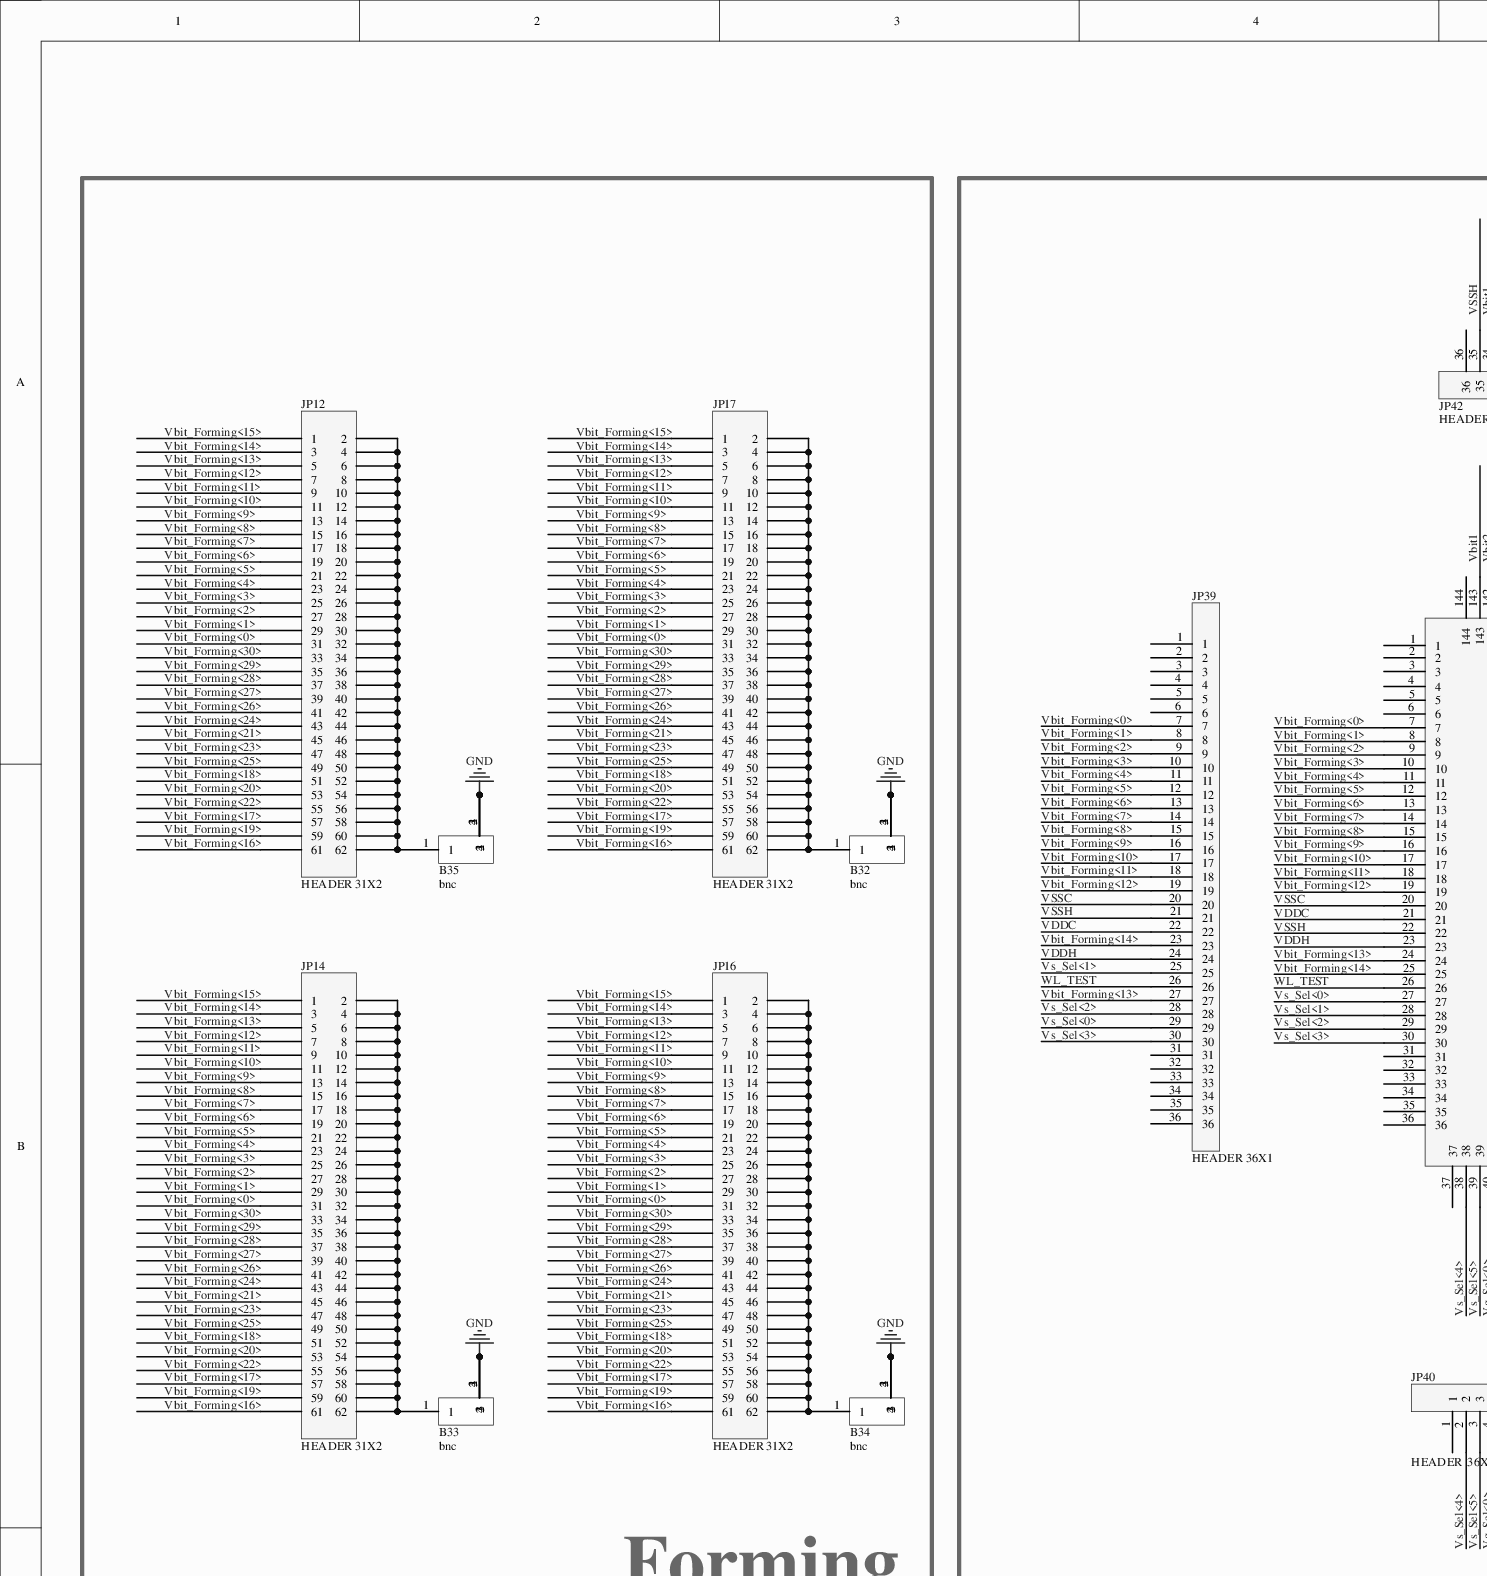
[diagram p0: MISC62794-8.SchDoc, top left]
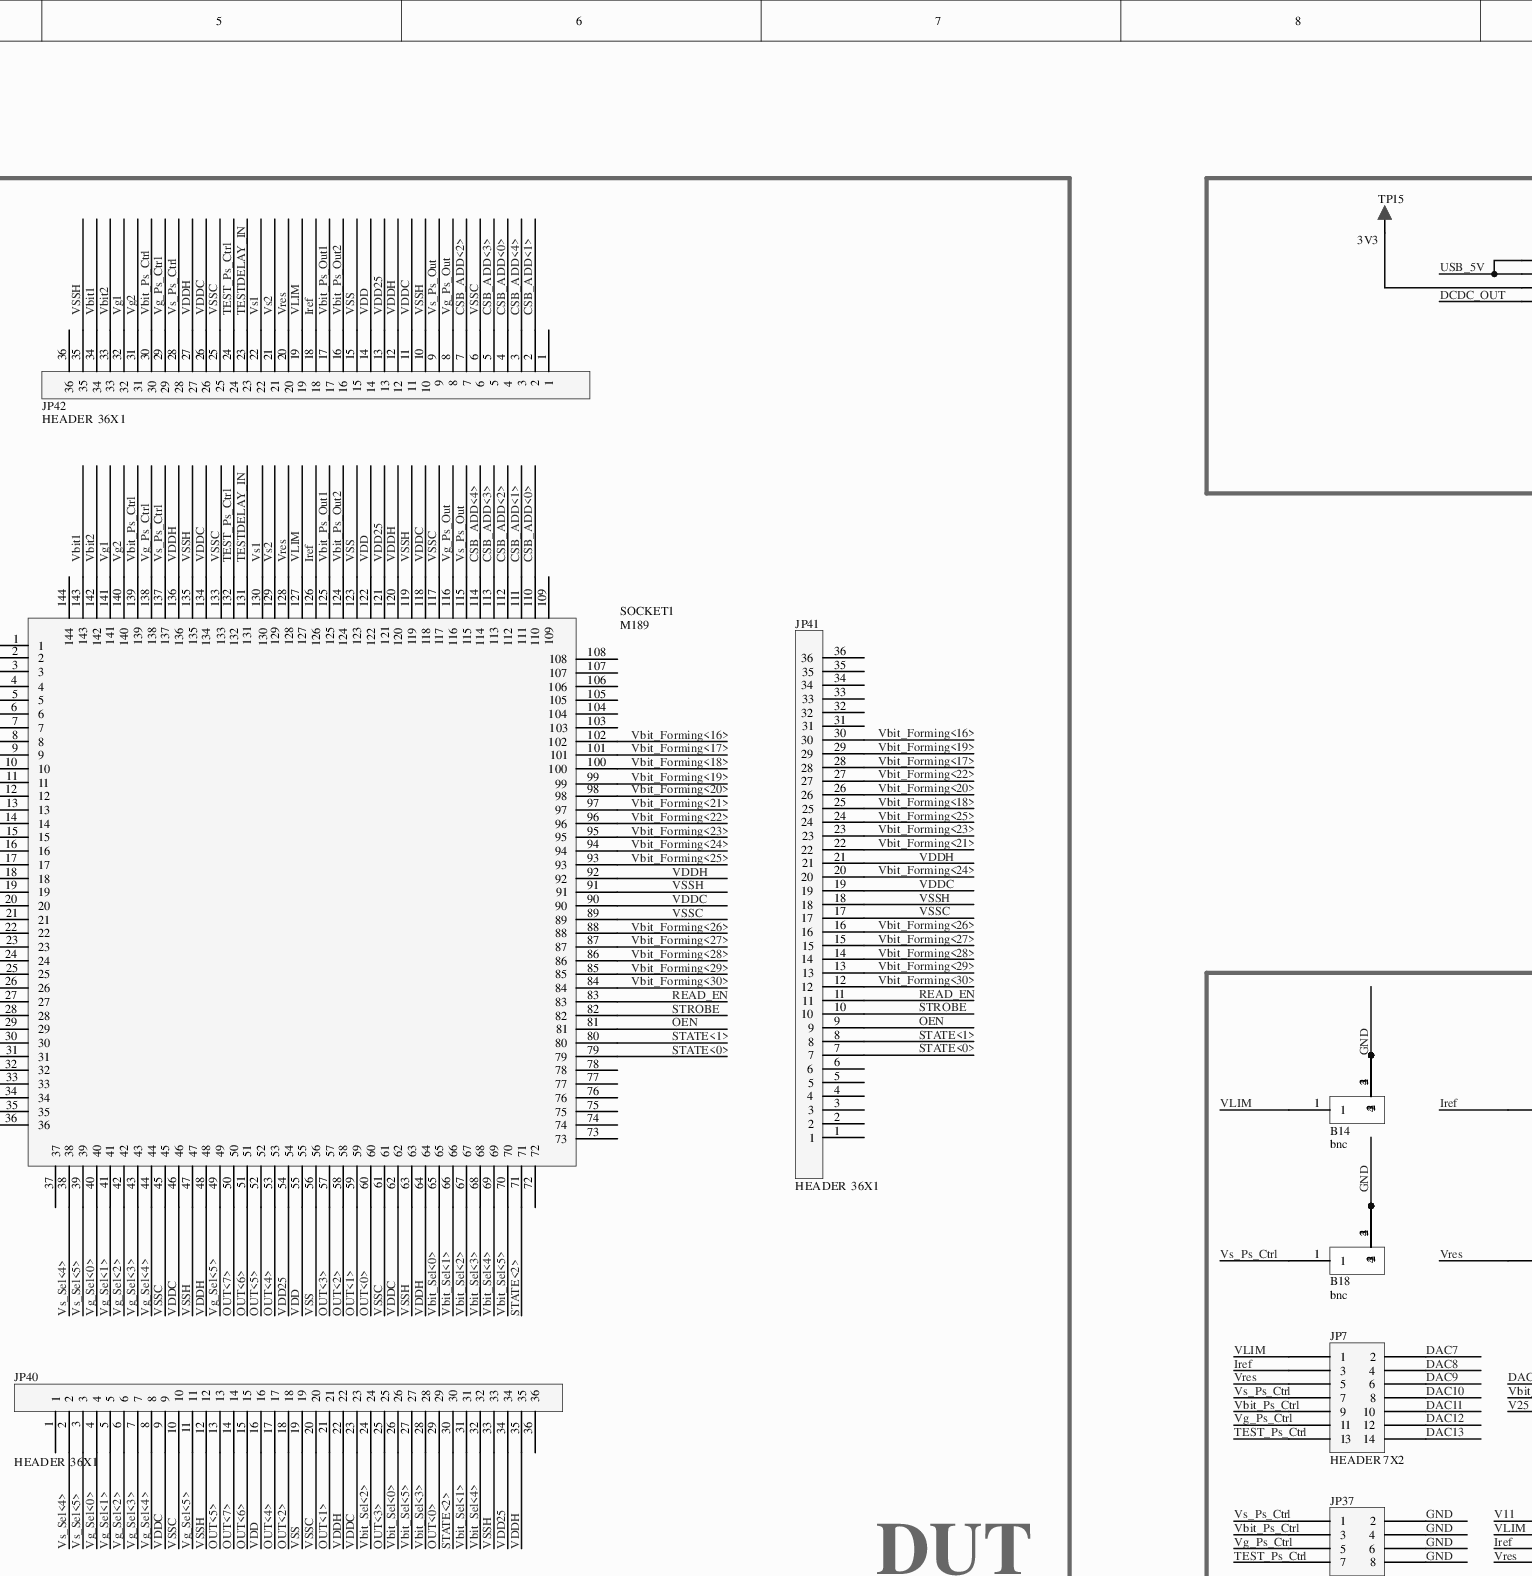
[diagram p1: MISC62794-8.SchDoc, top middle]
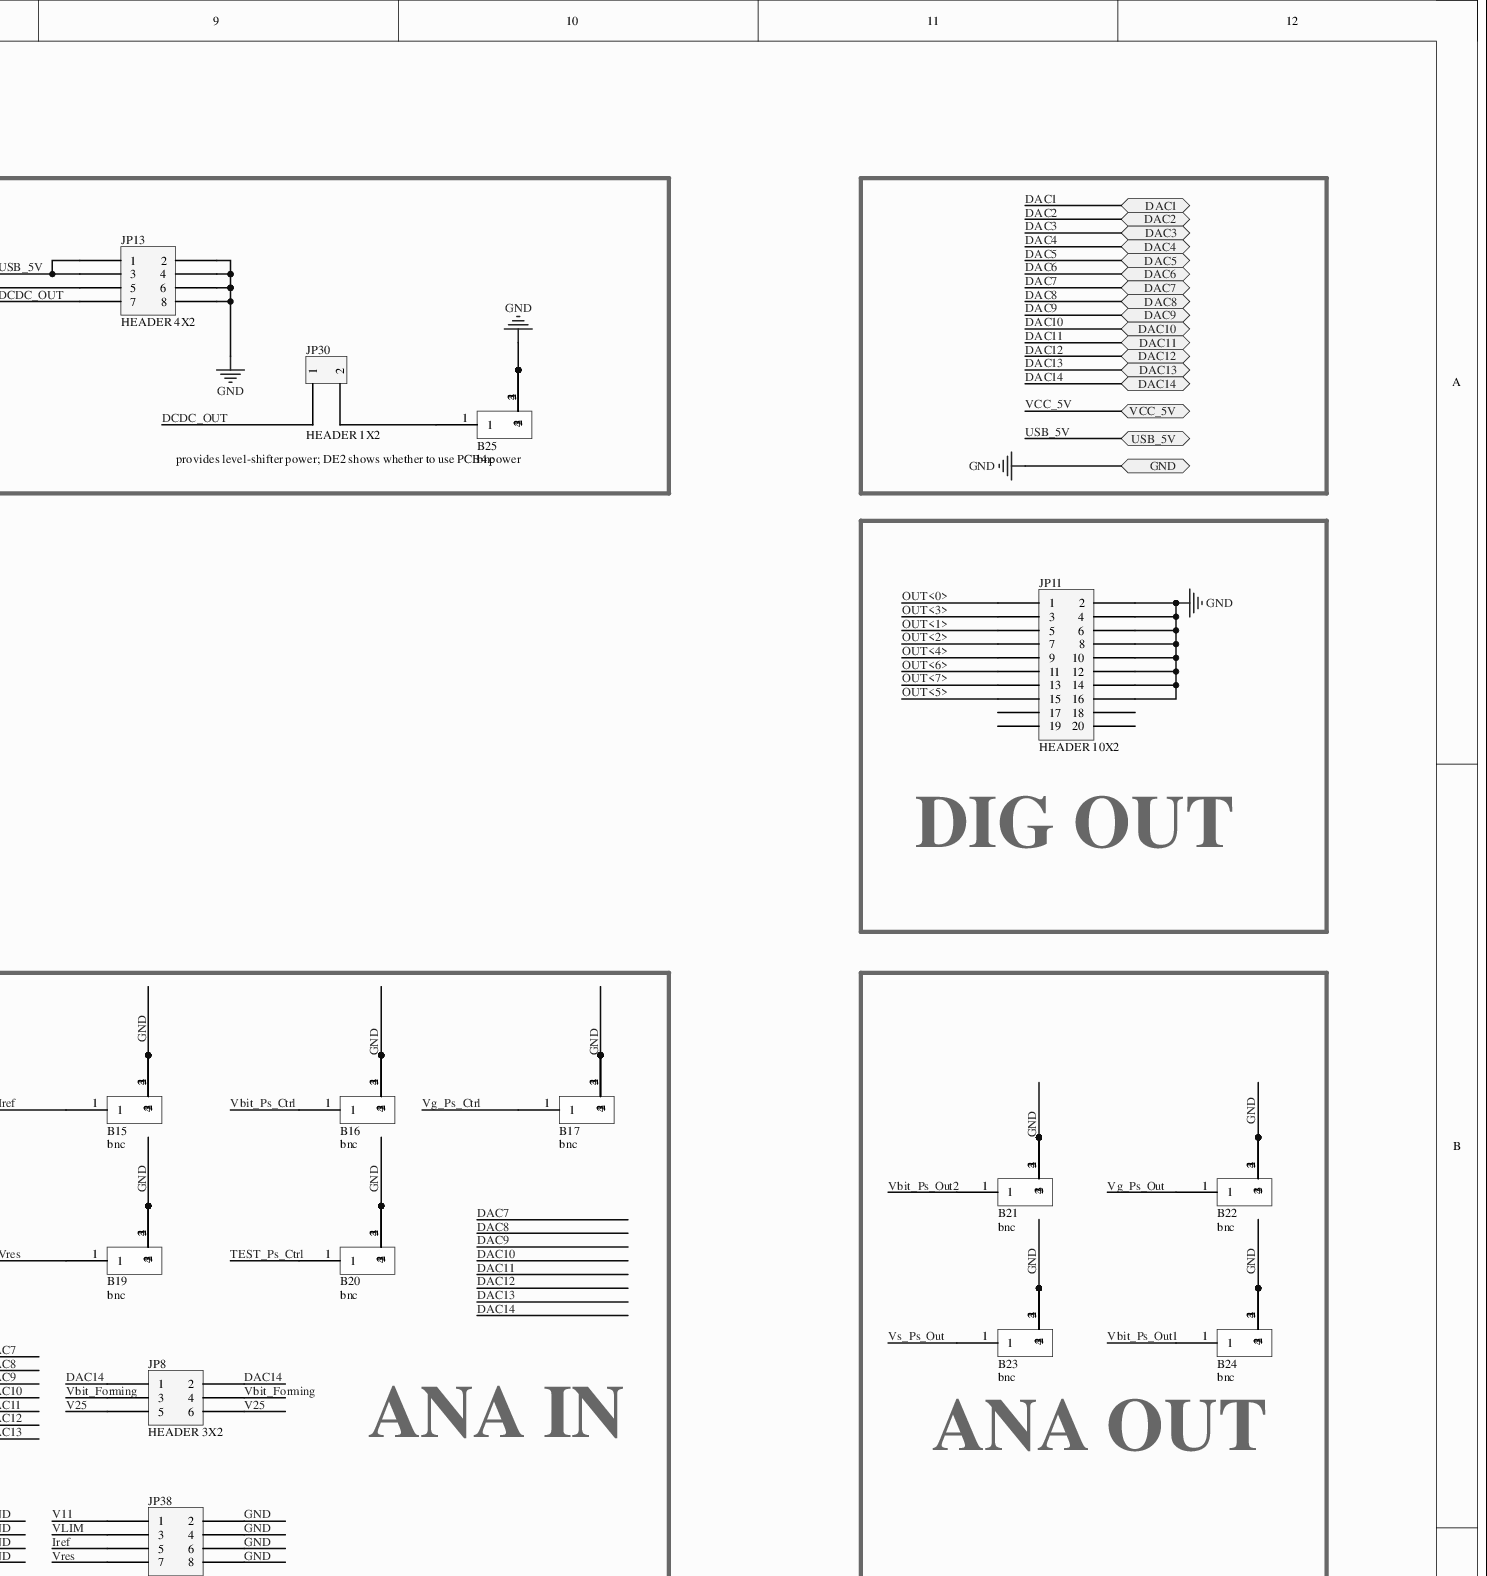
[diagram p2: MISC62794-8.SchDoc, top right]
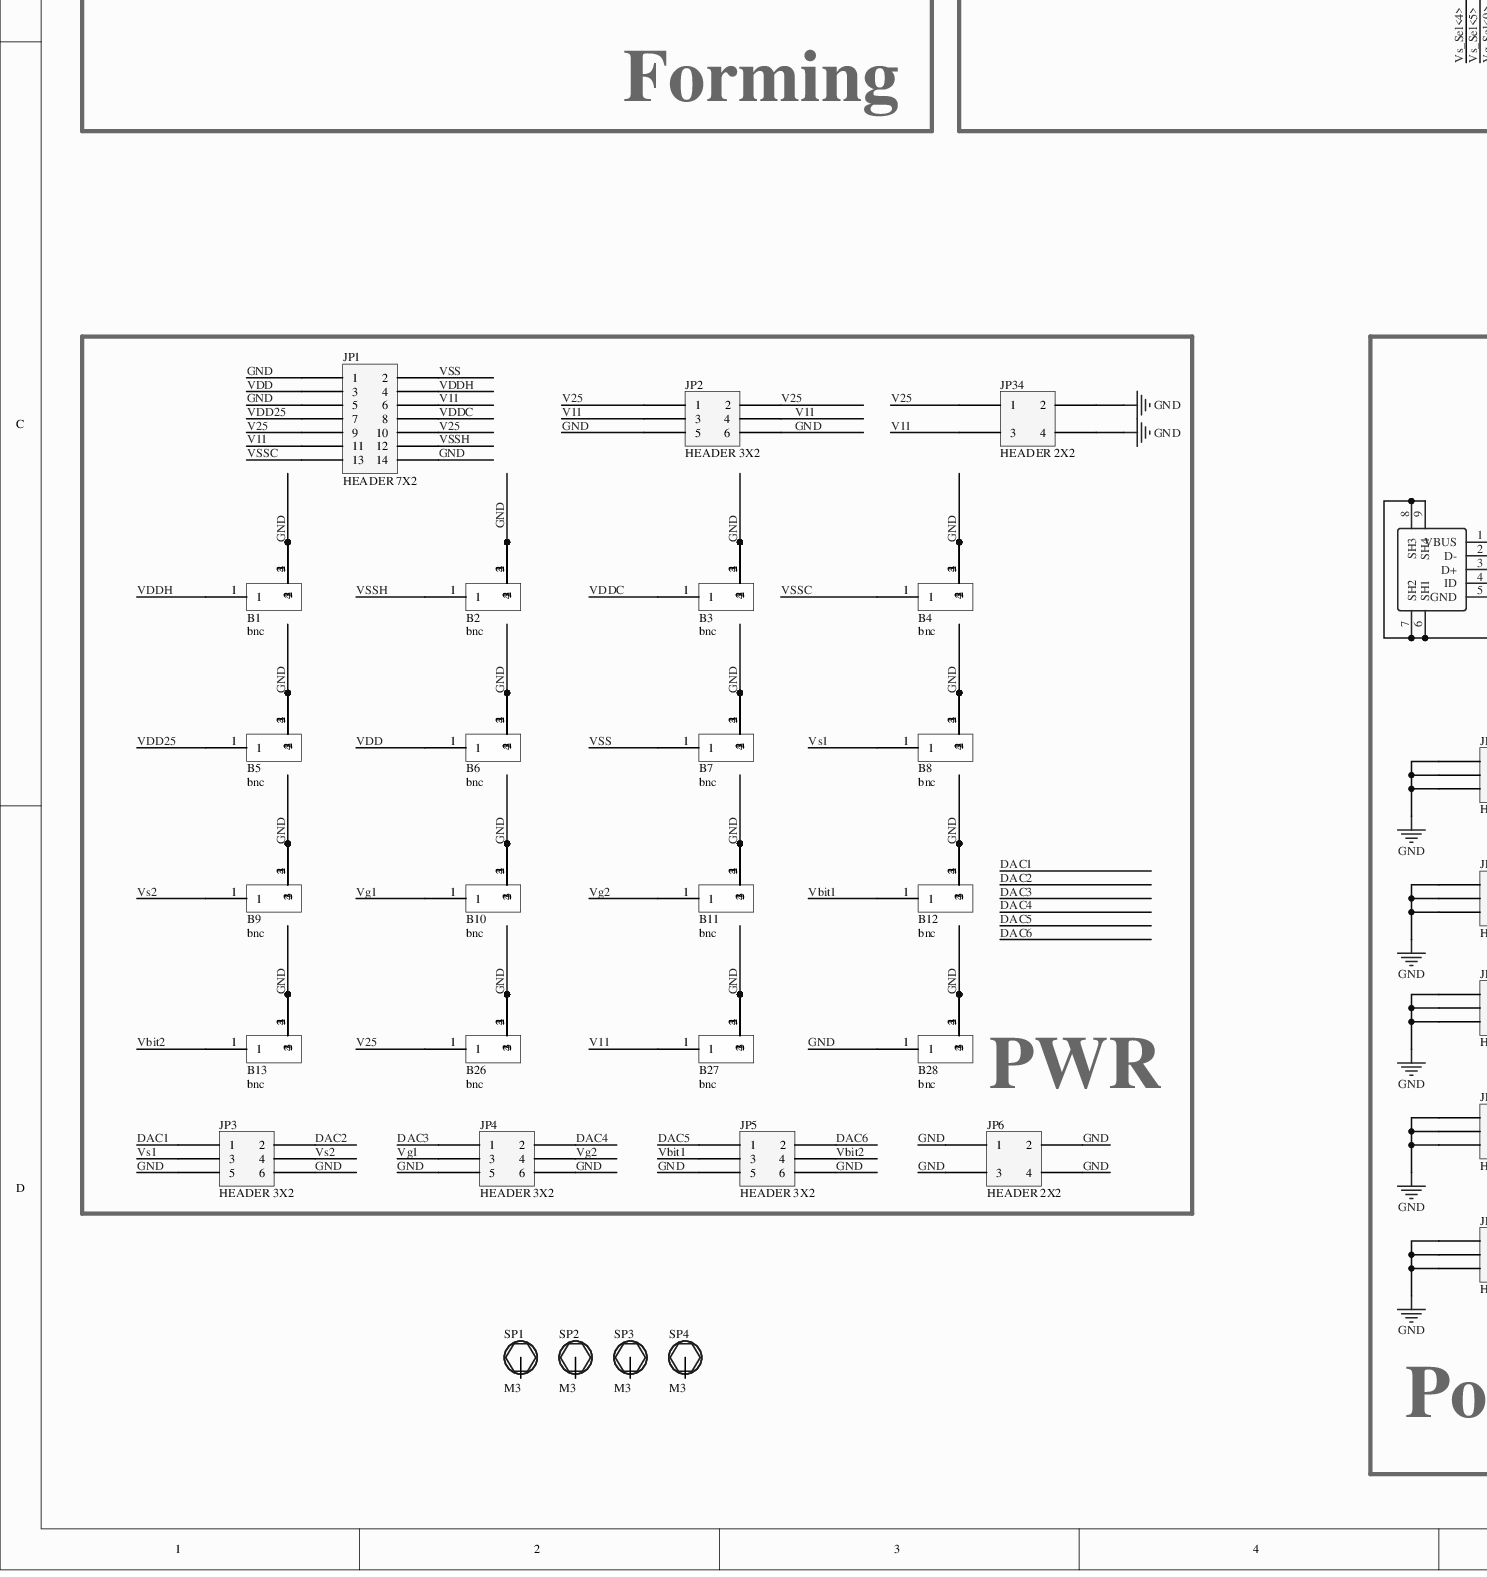
[diagram p3: MISC62794-8.SchDoc, bottom left]
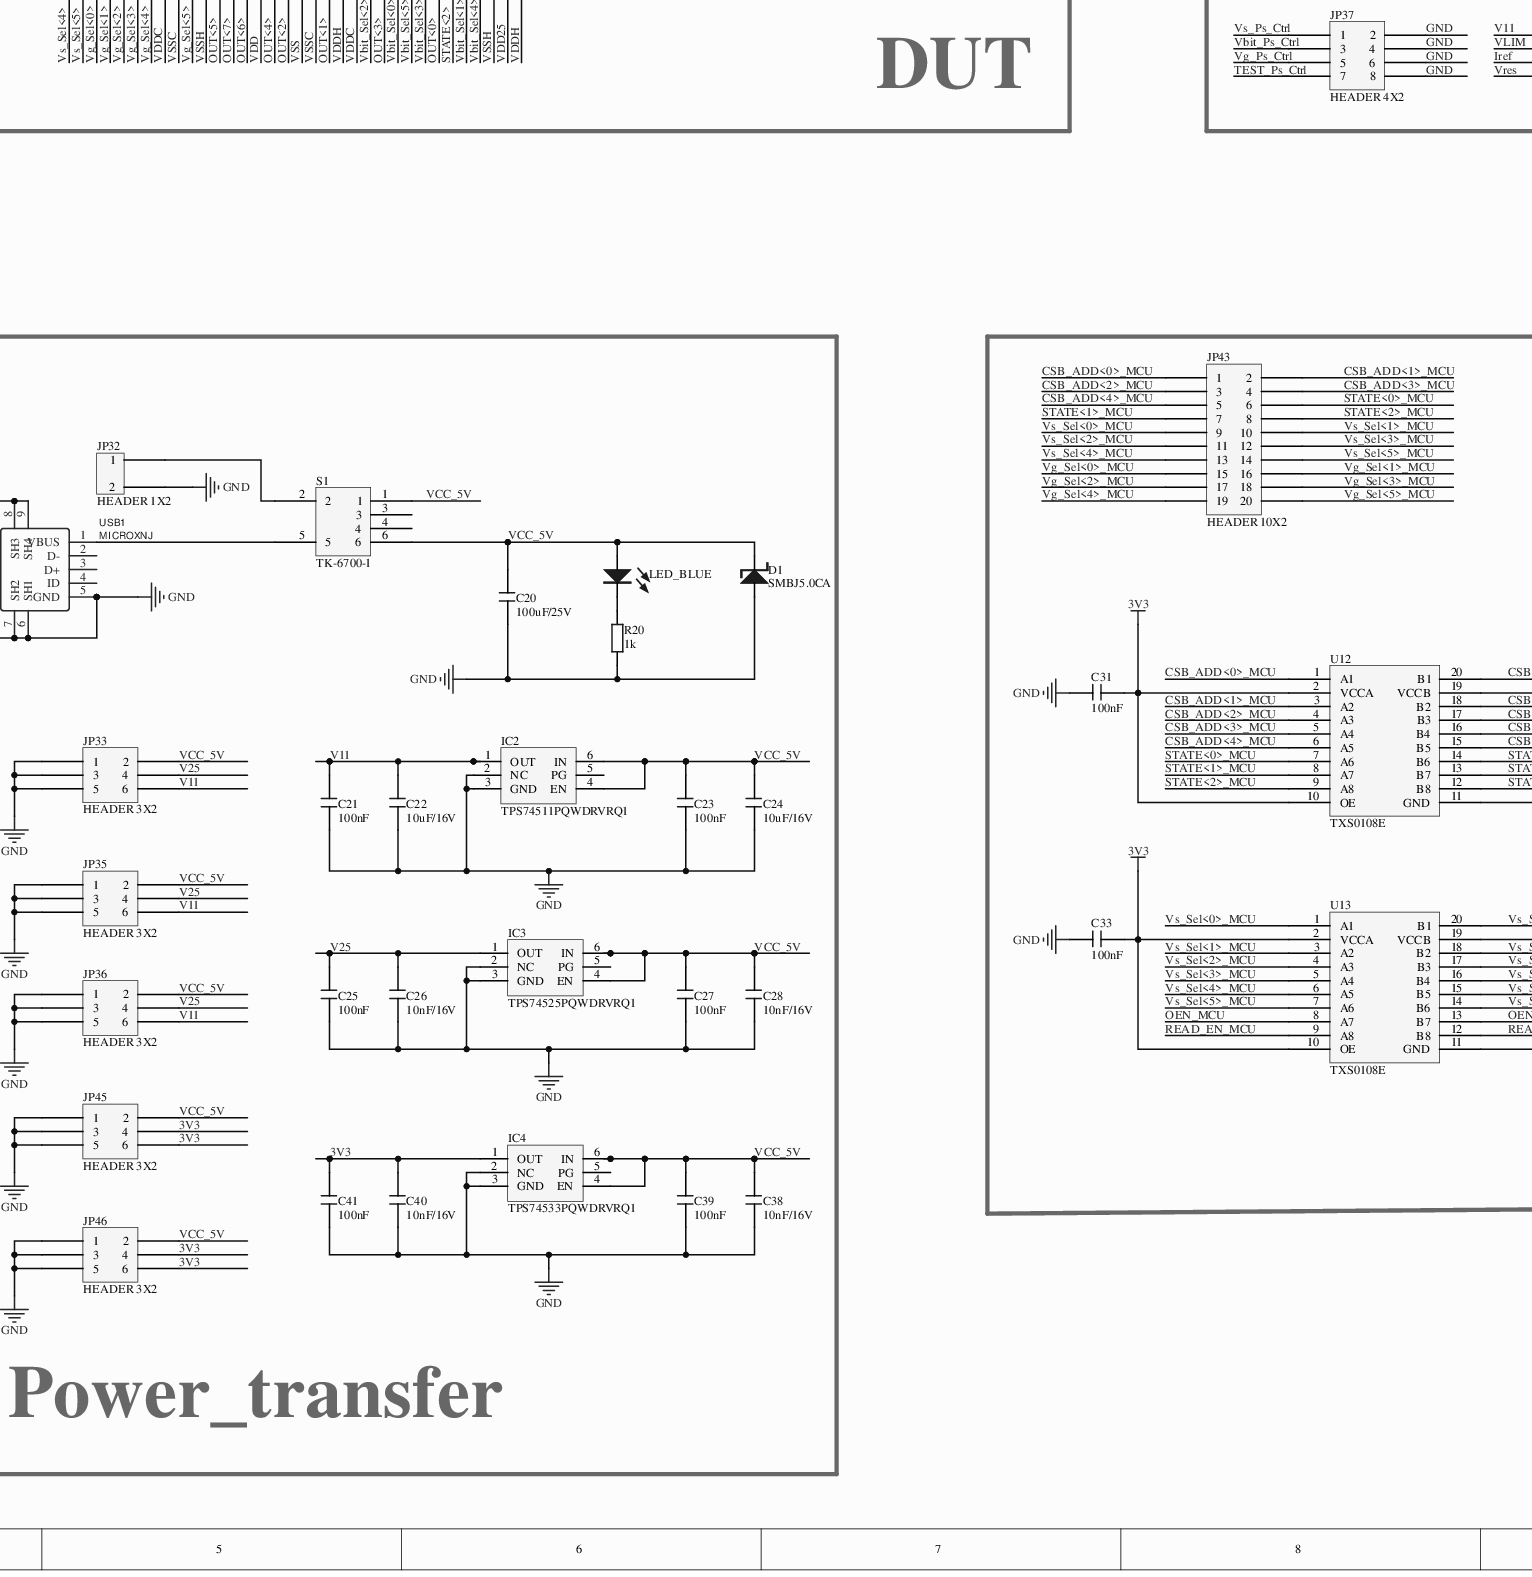
[diagram p4: MISC62794-8.SchDoc, bottom middle]
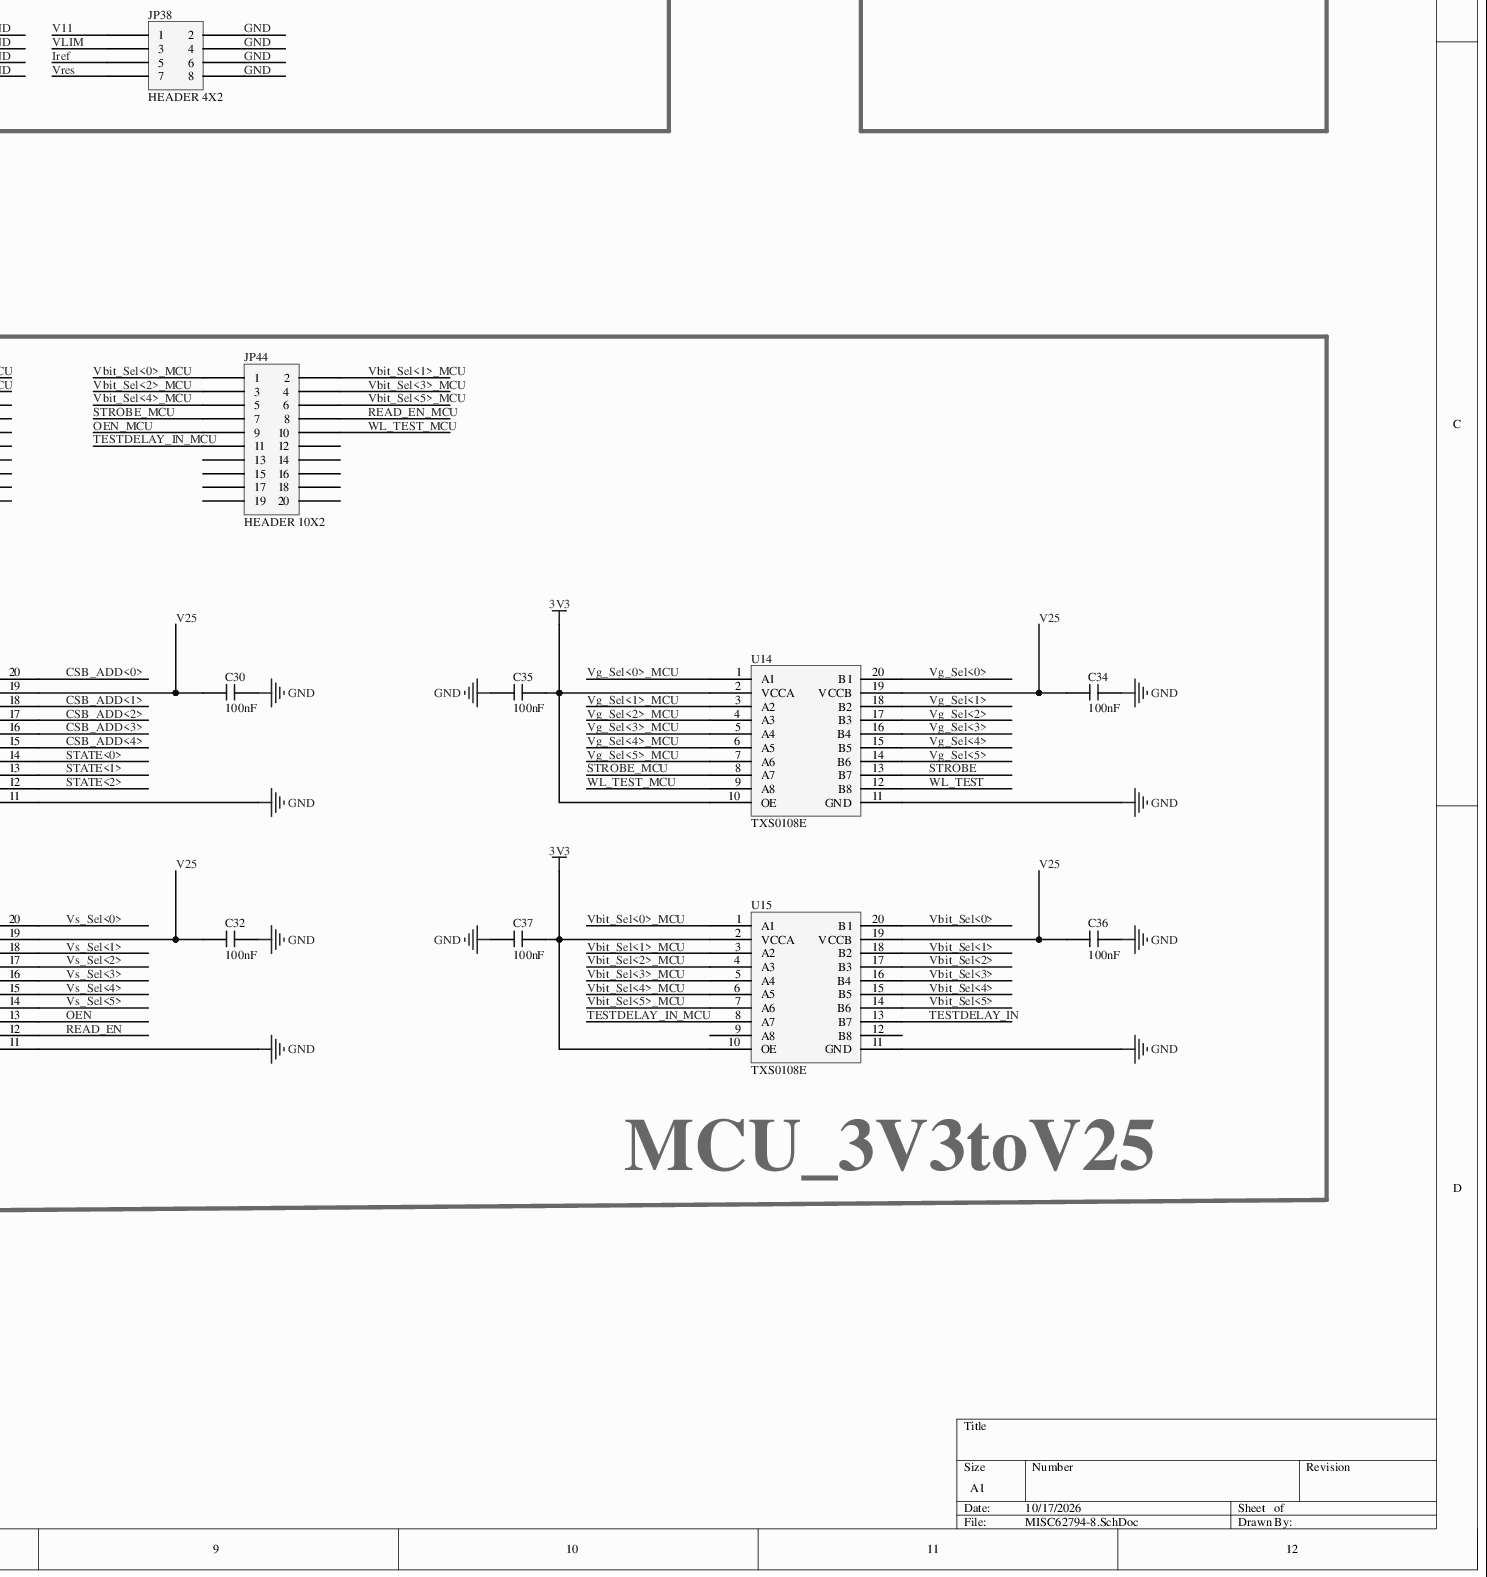
[diagram p5: MISC62794-8.SchDoc, bottom right]
# Altium project MISC62794-12.PrjPcb (part 2 of 3)

## Sheet MISC62794-8.SchDoc
size A1

### Parts
B1  bnc  [BNC-TH_DOSIN-801-0072]
B2  bnc  [BNC-TH_DOSIN-801-0072]
B3  bnc  [BNC-TH_DOSIN-801-0072]
B4  bnc  [BNC-TH_DOSIN-801-0072]
B5  bnc  [BNC-TH_DOSIN-801-0072]
B6  bnc  [BNC-TH_DOSIN-801-0072]
B7  bnc  [BNC-TH_DOSIN-801-0072]
B8  bnc  [BNC-TH_DOSIN-801-0072]
B9  bnc  [BNC-TH_DOSIN-801-0072]
B10  bnc  [BNC-TH_DOSIN-801-0072]
B11  bnc  [BNC-TH_DOSIN-801-0072]
B12  bnc  [BNC-TH_DOSIN-801-0072]
B13  bnc  [BNC-TH_DOSIN-801-0072]
B14  bnc  [BNC-TH_DOSIN-801-0072]
B15  bnc  [BNC-TH_DOSIN-801-0072]
B16  bnc  [BNC-TH_DOSIN-801-0072]
B17  bnc  [BNC-TH_DOSIN-801-0072]
B18  bnc  [BNC-TH_DOSIN-801-0072]
B19  bnc  [BNC-TH_DOSIN-801-0072]
B20  bnc  [BNC-TH_DOSIN-801-0072]
B21  bnc  [BNC-TH_DOSIN-801-0072]
B22  bnc  [BNC-TH_DOSIN-801-0072]
B23  bnc  [BNC-TH_DOSIN-801-0072]
B24  bnc  [BNC-TH_DOSIN-801-0072]
B25  bnc  [BNC-TH_DOSIN-801-0072]
B26  bnc  [BNC-TH_DOSIN-801-0072]
B27  bnc  [BNC-TH_DOSIN-801-0072]
B28  bnc  [BNC-TH_DOSIN-801-0072]
B32  bnc  [BNC-TH_DOSIN-801-0072]
B33  bnc  [BNC-TH_DOSIN-801-0072]
B34  bnc  [BNC-TH_DOSIN-801-0072]
B35  bnc  [BNC-TH_DOSIN-801-0072]
C20  100uF/25V  [EC-D6.3x7.7]
C21  100nF  [0603C]
C22  10uF/16V  [0603C]
C23  100nF  [0603C]
C24  10uF/16V  [0603C]
C25  100nF  [0603C]
C26  10nF/16V  [0603C]
C27  100nF  [0603C]
C28  10nF/16V  [0603C]
C30  100nF  [0603C]
C31  100nF  [0603C]
C32  100nF  [0603C]
C33  100nF  [0603C]
C34  100nF  [0603C]
C35  100nF  [0603C]
C36  100nF  [0603C]
C37  100nF  [0603C]
C38  10nF/16V  [0603C]
C39  100nF  [0603C]
C40  10nF/16V  [0603C]
C41  100nF  [0603C]
D1  SMBJ5.0CA  [SMB]
IC2  TPS74511PQWDRVRQ1  [WSON-6_L2.0-W2.0-P0.65-BL-EP]
IC3  TPS74525PQWDRVRQ1  [WSON-6_L2.0-W2.0-P0.65-BL-EP]
IC4  TPS74533PQWDRVRQ1  [WSON-6_L2.0-W2.0-P0.65-BL-EP]
JP1  HEADER 7X2  [HDR2.54-LI-2x7P]
JP2  HEADER 3X2  [HDR2.54-LI-2x3P]
JP3  HEADER 3X2  [HDR2.54-LI-2x3P]
JP4  HEADER 3X2  [HDR2.54-LI-2x3P]
JP5  HEADER 3X2  [HDR2.54-LI-2x3P]
JP6  HEADER 2X2  [HDR2.54-LI-2x3P]
JP7  HEADER 7X2  [HDR2.54-LI-2x7P]
JP8  HEADER 3X2  [HDR2.54-LI-2x3P]
JP11  HEADER 10X2  [HDR2.54-LI-2x10P]
JP12  HEADER 31X2  [HDR2.54-LI-2x31P]
JP13  HEADER 4X2  [HDR2.54-LI-2x4P]
JP14  HEADER 31X2  [HDR2.54-LI-2x31P]
JP16  HEADER 31X2  [HDR2.54-LI-2x31P]
JP17  HEADER 31X2  [HDR2.54-LI-2x31P]
JP30  HEADER 1X2  [HDR2.54-LI-2P]
JP32  HEADER 1X2  [HDR2.54-LI-2P]
JP33  HEADER 3X2  [HDR2.54-LI-2x3P]
JP34  HEADER 2X2  [HDR2.54-LI-2x2P]
JP35  HEADER 3X2  [HDR2.54-LI-2x3P]
JP36  HEADER 3X2  [HDR2.54-LI-2x3P]
JP37  HEADER 4X2  [HDR2.54-LI-2x4P]
JP38  HEADER 4X2  [HDR2.54-LI-2x4P]
JP39  HEADER 36X1  [HDR2.54-LI-1x36P]
JP40  HEADER  36X1  [HDR2.54-LI-1x36P]
JP41  HEADER  36X1  [HDR2.54-LI-1x36P]
JP42  HEADER  36X1  [HDR2.54-LI-1x36P]
JP43  HEADER 10X2  [HDR2.54-LI-2x10P]
JP44  HEADER 10X2  [HDR2.54-LI-2x10P]
JP45  HEADER 3X2  [HDR2.54-LI-2x3P]
JP46  HEADER 3X2  [HDR2.54-LI-2x3P]
LED_BLUE  LED  [LED0805-R-RD]  (value not drawn)
R20  1k  [0603R]
S1  TK-6700-1  [SW-TH_6P-L8.0-W8.0-P2.50]
SOCKET1  M189  [YAMAICHI_IC51-1444-1354-7]
SP1  M3  [M3]
SP2  M3  [M3]
SP3  M3  [M3]
SP4  M3  [M3]
TP15  3V3  [TP1.0]
U12  TXS0108E  [TSSOP-20_L6.5-W4.4-P0.65-LS6.4-BL]
U13  TXS0108E  [TSSOP-20_L6.5-W4.4-P0.65-LS6.4-BL]
U14  TXS0108E  [TSSOP-20_L6.5-W4.4-P0.65-LS6.4-BL]
U15  TXS0108E  [TSSOP-20_L6.5-W4.4-P0.65-LS6.4-BL]
USB1  MICROXNJ  [MICRO-USB-SMD_MICROXNJ]

### Ports
DAC1 (bidir), DAC2 (bidir), DAC3 (bidir), DAC4 (bidir), DAC5 (bidir), DAC6 (bidir), DAC7 (bidir), DAC8 (bidir), DAC9 (bidir), DAC10 (bidir), DAC11 (bidir), DAC12 (bidir), DAC13 (bidir), DAC14 (bidir), GND (bidir), USB_5V (bidir), VCC_5V (bidir)

### Nets
3V3: C31.1 C33.1 C35.1 C37.1 C40.1 C41.1 IC4.1(OUT) JP45.4 JP45.6 JP46.4 JP46.6 U12.2(VCCA) U12.10(OE) U13.2(VCCA) U13.10(OE) U14.2(VCCA) U14.10(OE) U15.2(VCCA) U15.10(OE)
GND: B1.2 B1.3 B1.4 B2.2 B2.3 B2.4 B3.2 B3.3 B3.4 B4.2 B4.3 B4.4 B5.2 B5.3 B5.4 B6.2 B6.3 B6.4 B7.2 B7.3 B7.4 B8.2 B8.3 B8.4 B9.2 B9.3 B9.4 B10.2 B10.3 B10.4 B11.2 B11.3 B11.4 B12.2 B12.3 B12.4 B13.2 B13.3 B13.4 B14.2 B14.3 B14.4 B15.2 B15.3 B15.4 B16.2 B16.3 B16.4 B17.2 B17.3 B17.4 B18.2 B18.3 B18.4 B19.2 B19.3 B19.4 B20.2 B20.3 B20.4 B21.2 B21.3 B21.4 B22.2 B22.3 B22.4 B23.2 B23.3 B23.4 B24.2 B24.3 B24.4 B25.2 B25.3 B25.4 B26.2 B26.3 B26.4 B27.2 B27.3 B27.4 B28.1 B28.2 B28.3 B28.4 B32.2 B32.3 B32.4 B33.2 B33.3 B33.4 B34.2 B34.3 B34.4 B35.2 B35.3 B35.4 C20.2 C21.2 C22.2 C23.2 C24.2 C25.2 C26.2 C27.2 C28.2 C30.1 C31.2 C32.1 C33.2 C34.1 C35.2 C36.1 C37.2 C38.2 C39.2 C40.2 C41.2 D1.2 IC2.2(NC) IC2.3(GND) IC3.2(NC) IC3.3(GND) IC4.2(NC) IC4.3(GND) JP1.1 JP1.5 JP1.14 JP2.5 JP2.6 JP3.5 JP3.6 JP4.5 JP4.6 JP5.5 JP5.6 JP6.1 JP6.2 JP6.3 JP6.4 JP11.2 JP11.4 JP11.6 JP11.8 JP11.10 JP11.12 JP11.14 JP11.16 JP13.2 JP13.4 JP13.6 JP13.8 JP32.2 JP33.1 JP33.3 JP33.5 JP34.2 JP34.4 JP35.1 JP35.3 JP35.5 JP36.1 JP36.3 JP36.5 JP37.2 JP37.4 JP37.6 JP37.8 JP38.2 JP38.4 JP38.6 JP38.8 JP45.1 JP45.3 JP45.5 JP46.1 JP46.3 JP46.5 R20.2 U12.11(GND) U13.11(GND) U14.11(GND) U15.11(GND) USB1.5(GND) USB1.6(SH1) USB1.7(SH2) USB1.8(SH3) USB1.9(SH4) ; port GND
USB_5V: JP13.1 JP13.3 ; port USB_5V
VCC_5V: C20.1 C23.1 C24.1 C27.1 C28.1 C38.1 C39.1 D1.1 IC2.4(EN) IC2.6(IN) IC3.4(EN) IC3.6(IN) IC4.4(EN) IC4.6(IN) JP33.2 JP35.2 JP36.2 JP45.2 JP46.2 LED_BLUE.1 S1.1 S1.6 ; port VCC_5V
CSB_ADD<0>: JP42.4 SOCKET1.110 U12.20(B1)
CSB_ADD<0>_MCU: JP43.1 U12.1(A1)
CSB_ADD<1>: JP42.2 SOCKET1.111 U12.18(B2)
CSB_ADD<1>_MCU: JP43.2 U12.3(A2)
CSB_ADD<2>: JP42.7 SOCKET1.112 U12.17(B3)
CSB_ADD<2>_MCU: JP43.3 U12.4(A3)
CSB_ADD<3>: JP42.5 SOCKET1.113 U12.16(B4)
CSB_ADD<3>_MCU: JP43.4 U12.5(A4)
CSB_ADD<4>: JP42.3 SOCKET1.114 U12.15(B5)
CSB_ADD<4>_MCU: JP43.5 U12.6(A5)
DAC1: JP3.1 ; port DAC1
DAC2: JP3.2 ; port DAC2
DAC3: JP4.1 ; port DAC3
DAC4: JP4.2 ; port DAC4
DAC5: JP5.1 ; port DAC5
DAC6: JP5.2 ; port DAC6
DAC7: JP7.2 ; port DAC7
DAC8: JP7.4 ; port DAC8
DAC9: JP7.6 ; port DAC9
DAC10: JP7.8 ; port DAC10
DAC11: JP7.10 ; port DAC11
DAC12: JP7.12 ; port DAC12
DAC13: JP7.14 ; port DAC13
DAC14: JP8.1 JP8.2 ; port DAC14
DCDC_OUT: JP13.7 JP30.1
Iref: B15.1 JP7.3 JP38.5 JP42.18 SOCKET1.126
OEN: JP41.9 SOCKET1.81 U13.13(B7)
OEN_MCU: JP44.9 U13.8(A7)
OUT<0>: JP11.1 JP40.29 SOCKET1.60
OUT<1>: JP11.5 JP40.21 SOCKET1.59
OUT<2>: JP11.7 JP40.18 SOCKET1.58
OUT<3>: JP11.3 JP40.25 SOCKET1.57
OUT<4>: JP11.9 JP40.17 SOCKET1.53
OUT<5>: JP11.15 JP40.13 SOCKET1.52
OUT<6>: JP11.11 JP40.15 SOCKET1.51
OUT<7>: JP11.13 JP40.14 SOCKET1.50
READ_EN: JP41.11 SOCKET1.83 U13.12(B8)
READ_EN_MCU: JP44.8 U13.9(A8)
STATE<0>: JP41.7 SOCKET1.79 U12.14(B6)
STATE<0>_MCU: JP43.6 U12.7(A6)
STATE<1>: JP41.8 SOCKET1.80 U12.13(B7)
STATE<1>_MCU: JP43.7 U12.8(A7)
STATE<2>: JP40.30 SOCKET1.71 U12.12(B8)
STATE<2>_MCU: JP43.8 U12.9(A8)
STROBE: JP41.10 SOCKET1.82 U14.13(B7)
STROBE_MCU: JP44.7 U14.8(A7)
TEST_Ps_Ctrl: B20.1 JP7.13 JP37.7 JP42.24 SOCKET1.132
TESTDELAY_IN: JP42.23 SOCKET1.131 U15.13(B7)
TESTDELAY_IN_MCU: JP44.11 U15.8(A7)
V11: B27.1 C21.1 C22.1 IC2.1(OUT) JP1.6 JP1.11 JP2.3 JP2.4 JP33.6 JP34.3 JP35.6 JP36.6 JP38.1
V25: B26.1 C25.1 C26.1 C30.2 C32.2 C34.2 C36.2 IC3.1(OUT) JP1.9 JP1.10 JP2.1 JP2.2 JP8.5 JP8.6 JP33.4 JP34.1 JP35.4 JP36.4 U12.19(VCCB) U13.19(VCCB) U14.19(VCCB) U15.19(VCCB)
Vbit1: B12.1 JP5.3 JP42.34 SOCKET1.143
Vbit2: B13.1 JP5.4 JP42.33 SOCKET1.142
Vbit_Forming: JP8.3 JP8.4
Vbit_Forming<0>: JP12.31 JP14.31 JP16.31 JP17.31 JP39.7 SOCKET1.7
Vbit_Forming<1>: JP12.29 JP14.29 JP16.29 JP17.29 JP39.8 SOCKET1.8
Vbit_Forming<2>: JP12.27 JP14.27 JP16.27 JP17.27 JP39.9 SOCKET1.9
Vbit_Forming<3>: JP12.25 JP14.25 JP16.25 JP17.25 JP39.10 SOCKET1.10
Vbit_Forming<4>: JP12.23 JP14.23 JP16.23 JP17.23 JP39.11 SOCKET1.11
Vbit_Forming<5>: JP12.21 JP14.21 JP16.21 JP17.21 JP39.12 SOCKET1.12
Vbit_Forming<6>: JP12.19 JP14.19 JP16.19 JP17.19 JP39.13 SOCKET1.13
Vbit_Forming<7>: JP12.17 JP14.17 JP16.17 JP17.17 JP39.14 SOCKET1.14
Vbit_Forming<8>: JP12.15 JP14.15 JP16.15 JP17.15 JP39.15 SOCKET1.15
Vbit_Forming<9>: JP12.13 JP14.13 JP16.13 JP17.13 JP39.16 SOCKET1.16
Vbit_Forming<10>: JP12.11 JP14.11 JP16.11 JP17.11 JP39.17 SOCKET1.17
Vbit_Forming<11>: JP12.9 JP14.9 JP16.9 JP17.9 JP39.18 SOCKET1.18
Vbit_Forming<12>: JP12.7 JP14.7 JP16.7 JP17.7 JP39.19 SOCKET1.19
Vbit_Forming<13>: JP12.5 JP14.5 JP16.5 JP17.5 JP39.27 SOCKET1.24
Vbit_Forming<14>: JP12.3 JP14.3 JP16.3 JP17.3 JP39.23 SOCKET1.25
Vbit_Forming<15>: JP12.1 JP14.1 JP16.1 JP17.1
Vbit_Forming<16>: JP12.61 JP14.61 JP16.61 JP17.61 JP41.30 SOCKET1.102
Vbit_Forming<17>: JP12.57 JP14.57 JP16.57 JP17.57 JP41.28 SOCKET1.101
Vbit_Forming<18>: JP12.51 JP14.51 JP16.51 JP17.51 JP41.25 SOCKET1.100
Vbit_Forming<19>: JP12.59 JP14.59 JP16.59 JP17.59 JP41.29 SOCKET1.99
Vbit_Forming<20>: JP12.53 JP14.53 JP16.53 JP17.53 JP41.26 SOCKET1.98
Vbit_Forming<21>: JP12.45 JP14.45 JP16.45 JP17.45 JP41.22 SOCKET1.97
Vbit_Forming<22>: JP12.55 JP14.55 JP16.55 JP17.55 JP41.27 SOCKET1.96
Vbit_Forming<23>: JP12.47 JP14.47 JP16.47 JP17.47 JP41.23 SOCKET1.95
Vbit_Forming<24>: JP12.43 JP14.43 JP16.43 JP17.43 JP41.20 SOCKET1.94
Vbit_Forming<25>: JP12.49 JP14.49 JP16.49 JP17.49 JP41.24 SOCKET1.93
Vbit_Forming<26>: JP12.41 JP14.41 JP16.41 JP17.41 JP41.16 SOCKET1.88
Vbit_Forming<27>: JP12.39 JP14.39 JP16.39 JP17.39 JP41.15 SOCKET1.87
Vbit_Forming<28>: JP12.37 JP14.37 JP16.37 JP17.37 JP41.14 SOCKET1.86
Vbit_Forming<29>: JP12.35 JP14.35 JP16.35 JP17.35 JP41.13 SOCKET1.85
Vbit_Forming<30>: JP12.33 JP14.33 JP16.33 JP17.33 JP41.12 SOCKET1.84
Vbit_Ps_Ctrl: B16.1 JP7.9 JP37.3 JP42.30 SOCKET1.139
Vbit_Ps_Out1: B24.1 JP42.17 SOCKET1.125
Vbit_Ps_Out2: B21.1 JP42.16 SOCKET1.124
Vbit_Sel<0>: JP40.26 SOCKET1.65 U15.20(B1)
Vbit_Sel<0>_MCU: JP44.1 U15.1(A1)
Vbit_Sel<1>: JP40.31 SOCKET1.66 U15.18(B2)
Vbit_Sel<1>_MCU: JP44.2 U15.3(A2)
Vbit_Sel<2>: JP40.24 SOCKET1.67 U15.17(B3)
Vbit_Sel<2>_MCU: JP44.3 U15.4(A3)
Vbit_Sel<3>: JP40.28 SOCKET1.68 U15.16(B4)
Vbit_Sel<3>_MCU: JP44.4 U15.5(A4)
Vbit_Sel<4>: JP40.32 SOCKET1.69 U15.15(B5)
Vbit_Sel<4>_MCU: JP44.5 U15.6(A5)
Vbit_Sel<5>: JP40.27 SOCKET1.70 U15.14(B6)
Vbit_Sel<5>_MCU: JP44.6 U15.7(A6)
VDD: B6.1 JP1.3 JP40.16 JP42.14 SOCKET1.55 SOCKET1.122
VDD25: B5.1 JP1.7 JP40.34 JP42.13 SOCKET1.54 SOCKET1.121
VDDC: B3.1 JP1.8 JP39.22 JP40.9 JP40.23 JP41.19 JP42.11 JP42.26 SOCKET1.21 SOCKET1.46 SOCKET1.62 SOCKET1.90 SOCKET1.118 SOCKET1.134
VDDH: B1.1 JP1.4 JP39.24 JP40.22 JP40.35 JP41.21 JP42.12 JP42.27 SOCKET1.23 SOCKET1.48 SOCKET1.64 SOCKET1.92 SOCKET1.120 SOCKET1.136
Vg1: B10.1 JP4.3 JP42.32 SOCKET1.141
Vg2: B11.1 JP4.4 JP42.31 SOCKET1.140
Vg_Ps_Ctrl: B17.1 JP7.11 JP37.5 JP42.29 SOCKET1.138
Vg_Ps_Out: B22.1 JP42.8 SOCKET1.116
Vg_Sel<0>: JP40.4 SOCKET1.40 U14.20(B1)
Vg_Sel<0>_MCU: JP43.15 U14.1(A1)
Vg_Sel<1>: JP40.5 SOCKET1.41 U14.18(B2)
Vg_Sel<1>_MCU: JP43.16 U14.3(A2)
Vg_Sel<2>: JP40.6 SOCKET1.42 U14.17(B3)
Vg_Sel<2>_MCU: JP43.17 U14.4(A3)
Vg_Sel<3>: JP40.7 SOCKET1.43 U14.16(B4)
Vg_Sel<3>_MCU: JP43.18 U14.5(A4)
Vg_Sel<4>: JP40.8 SOCKET1.44 U14.15(B5)
Vg_Sel<4>_MCU: JP43.19 U14.6(A5)
Vg_Sel<5>: JP40.11 SOCKET1.49 U14.14(B6)
Vg_Sel<5>_MCU: JP43.20 U14.7(A6)
VLIM: B14.1 JP7.1 JP38.3 JP42.19 SOCKET1.127
Vres: B19.1 JP7.5 JP38.7 JP42.20 SOCKET1.128
Vs1: B8.1 JP3.3 JP42.22 SOCKET1.130
Vs2: B9.1 JP3.4 JP42.21 SOCKET1.129
Vs_Ps_Ctrl: B18.1 JP7.7 JP37.1 JP42.28 SOCKET1.137
Vs_Ps_Out: B23.1 JP42.9 SOCKET1.115
Vs_Sel<0>: JP39.29 SOCKET1.27 U13.20(B1)
Vs_Sel<0>_MCU: JP43.9 U13.1(A1)
Vs_Sel<1>: JP39.25 SOCKET1.28 U13.18(B2)
Vs_Sel<1>_MCU: JP43.10 U13.3(A2)
Vs_Sel<2>: JP39.28 SOCKET1.29 U13.17(B3)
Vs_Sel<2>_MCU: JP43.11 U13.4(A3)
Vs_Sel<3>: JP39.30 SOCKET1.30 U13.16(B4)
Vs_Sel<3>_MCU: JP43.12 U13.5(A4)
Vs_Sel<4>: JP40.2 SOCKET1.38 U13.15(B5)
Vs_Sel<4>_MCU: JP43.13 U13.6(A5)
Vs_Sel<5>: JP40.3 SOCKET1.39 U13.14(B6)
Vs_Sel<5>_MCU: JP43.14 U13.7(A6)
VSS: B7.1 JP1.2 JP40.19 JP42.15 SOCKET1.56 SOCKET1.123
VSSC: B4.1 JP1.13 JP39.20 JP40.10 JP40.20 JP41.17 JP42.6 JP42.25 SOCKET1.20 SOCKET1.45 SOCKET1.61 SOCKET1.89 SOCKET1.117 SOCKET1.133
VSSH: B2.1 JP1.12 JP39.21 JP40.12 JP40.33 JP41.18 JP42.10 JP42.35 SOCKET1.22 SOCKET1.47 SOCKET1.63 SOCKET1.91 SOCKET1.119 SOCKET1.135
WL_TEST: JP39.26 SOCKET1.26 U14.12(B8)
WL_TEST_MCU: JP44.10 U14.9(A8)
NetB25_1: B25.1 JP30.2
NetB32_1: B32.1 JP17.2 JP17.4 JP17.6 JP17.8 JP17.10 JP17.12 JP17.14 JP17.16 JP17.18 JP17.20 JP17.22 JP17.24 JP17.26 JP17.28 JP17.30 JP17.32 JP17.34 JP17.36 JP17.38 JP17.40 JP17.42 JP17.44 JP17.46 JP17.48 JP17.50 JP17.52 JP17.54 JP17.56 JP17.58 JP17.60 JP17.62
NetB33_1: B33.1 JP14.2 JP14.4 JP14.6 JP14.8 JP14.10 JP14.12 JP14.14 JP14.16 JP14.18 JP14.20 JP14.22 JP14.24 JP14.26 JP14.28 JP14.30 JP14.32 JP14.34 JP14.36 JP14.38 JP14.40 JP14.42 JP14.44 JP14.46 JP14.48 JP14.50 JP14.52 JP14.54 JP14.56 JP14.58 JP14.60 JP14.62
NetB34_1: B34.1 JP16.2 JP16.4 JP16.6 JP16.8 JP16.10 JP16.12 JP16.14 JP16.16 JP16.18 JP16.20 JP16.22 JP16.24 JP16.26 JP16.28 JP16.30 JP16.32 JP16.34 JP16.36 JP16.38 JP16.40 JP16.42 JP16.44 JP16.46 JP16.48 JP16.50 JP16.52 JP16.54 JP16.56 JP16.58 JP16.60 JP16.62
NetB35_1: B35.1 JP12.2 JP12.4 JP12.6 JP12.8 JP12.10 JP12.12 JP12.14 JP12.16 JP12.18 JP12.20 JP12.22 JP12.24 JP12.26 JP12.28 JP12.30 JP12.32 JP12.34 JP12.36 JP12.38 JP12.40 JP12.42 JP12.44 JP12.46 JP12.48 JP12.50 JP12.52 JP12.54 JP12.56 JP12.58 JP12.60 JP12.62
NetJP13_5: JP13.5 TP15.1
NetJP32_1: JP32.1 S1.2
NetLED_BLUE_2: LED_BLUE.2 R20.1
NetS1_5: S1.5 USB1.1(VBUS)

Not connected (* = marked no-connect by the designer): IC2 5(PG); IC3 5(PG); IC4 5(PG); JP11 17 18 19 20; JP39 1 2 3 4 5 6 31 32 33 34 35 36; JP40 1 36; JP41 1 2 3 4 5 6 31 32 33 34 35 36; JP42 1 36; JP44 12 13 14 15 16 17 18 19 20; S1 3 4; SOCKET1 1 2 3 4 5 6 31 32 33 34 35 36 37 72 73 74 75 76 77 78 103 104 105 106 107 108 109 144; SP1 1; SP2 1; SP3 1; SP4 1; U15 9(A8)* 12(B8)*; USB1 2(D-) 3(D+) 4(ID)

### Notes on the sheet
- (near B25) provides level-shifter power; DE2 shows whether to use PCB4 power
- DIG OUT
- ANA IN
- ANA OUT
- Forming
- DUT
- (near B28) PWR
- MCU_3V3toV25
- Power_transfer

### Library data of the parts
C20-C28 C30-C41 = CAP: capacitor model
D1 = SMBJ5.0CA: diode
IC2 = TPS74511PQWDRVRQ1: LDO
IC3 = TPS74525PQWDRVRQ1: LDO
IC4 = TPS74533PQWDRVRQ1: LDO
JP1 JP7 = HEADER 7X2: pin header
JP2-JP5 JP8 JP33 JP35 JP36 JP45 JP46 = HEADER 3X2: pin header
JP6 JP34 = HEADER 2X2: pin header
JP11 JP43 JP44 = HEADER 10X2: pin header
JP12 JP14 JP16 JP17 = HEADER 31X2: pin header
JP13 JP37 JP38 = HEADER 4X2: pin header
JP30 JP32 = HEADER 1X2: pin header
JP39-JP42 = HEADER 36X1: pin header
LED_BLUE = LED: light-emitting diode
R20 = RES: resistor model
S1 = switch6: six-pin self-locking switch
SOCKET1 = M189_4K: array
SP1-SP4 = M3: M3 interface
TP15 = TP